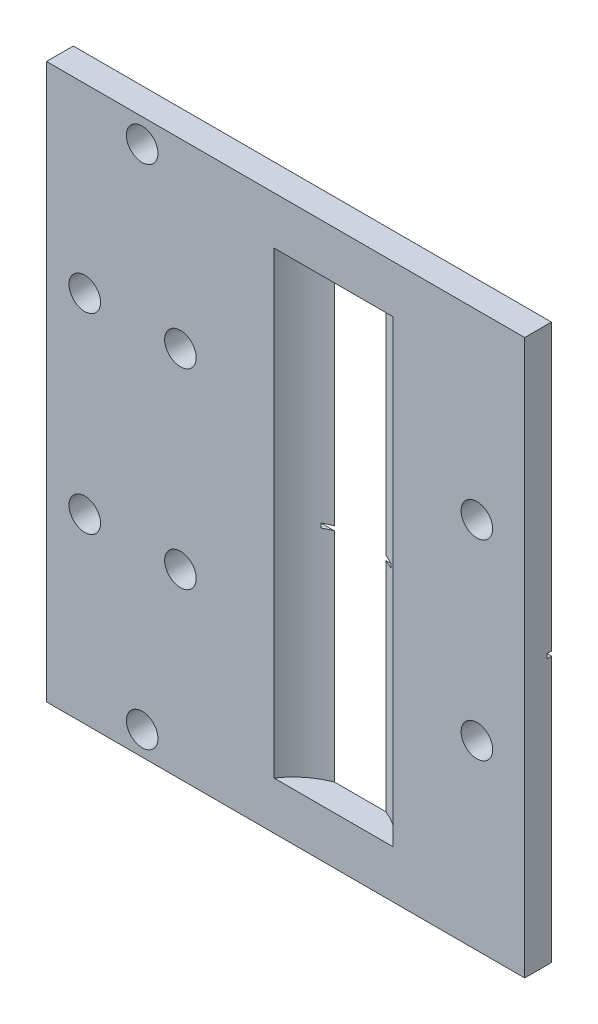
from build123d import *

# Parameters (mm, degrees)
SKETCH_1_W          = 50
SKETCH_1_H          = 58
EXTRUDE_1_DEPTH     = 2.8
SKETCH_2_R          = 1.65
CUT_EXTRUDE_1_DEPTH = 54.537707789
SKETCH_3_W          = 0.45
SKETCH_3_H          = 0.45
CUT_EXTRUDE_2_DEPTH = 63.005437899
CUT_EXTRUDE_3_DEPTH = 48


with BuildPart() as part:
    # 草图1 → 凸台-拉伸1 (new body)
    with BuildSketch(Plane.XY):
        with Locations((-14.007843137, -7.562745098)):
            Rectangle(SKETCH_1_W, SKETCH_1_H)
    extrude(amount=EXTRUDE_1_DEPTH)

    # 草图2 → 切除-拉伸1 (cut, through all)
    with BuildSketch(Plane.XY.offset(2.8)):
        with Locations((-29.007843137, 18.937254902)):
            Circle(SKETCH_2_R)
        with Locations((-35.007843137, 2.437254902)):
            Circle(SKETCH_2_R)
        with Locations((-25.007843137, 2.437254902)):
            Circle(SKETCH_2_R)
        with Locations((5.992156863, 2.437254902)):
            Circle(SKETCH_2_R)
        with Locations((-35.007843137, -17.562745098)):
            Circle(SKETCH_2_R)
        with Locations((-25.007843137, -17.562745098)):
            Circle(SKETCH_2_R)
        with Locations((-29.007843137, -34.062745098)):
            Circle(SKETCH_2_R)
        with Locations((5.992156863, -17.562745098)):
            Circle(SKETCH_2_R)
    extrude(amount=-CUT_EXTRUDE_1_DEPTH, mode=Mode.SUBTRACT)

    # 草图3 → 切除-拉伸2 (cut, through all)
    with BuildSketch(Plane(origin=(10.992156863, 0, 0), x_dir=(0, 0, -1), z_dir=(1, 0, 0))):
        with Locations((-0.225, -8.587745098)):
            Rectangle(SKETCH_3_W, SKETCH_3_H)
    extrude(amount=-CUT_EXTRUDE_2_DEPTH, mode=Mode.SUBTRACT)

    # 草图5 → 切除-拉伸3 (cut)
    with BuildSketch(Plane(origin=(0, 16.437254902, 0), x_dir=(1, 0, 0), z_dir=(0, 1, 0))):
        with BuildLine():
            Line((-2.794148584, -2.8), (-15.22153769, -2.8))
            ThreePointArc((-15.22153769, -2.8), (-13.675866521, -1.129773625), (-11.700425541, 0))
            Line((-11.700425541, 0), (-6.408228111, 0.035055203))
            ThreePointArc((-6.408228111, 0.035055203), (-4.378805339, -1.098982371), (-2.794148584, -2.8))
        make_face()
    extrude(amount=-CUT_EXTRUDE_3_DEPTH, mode=Mode.SUBTRACT)


solid = part.part
